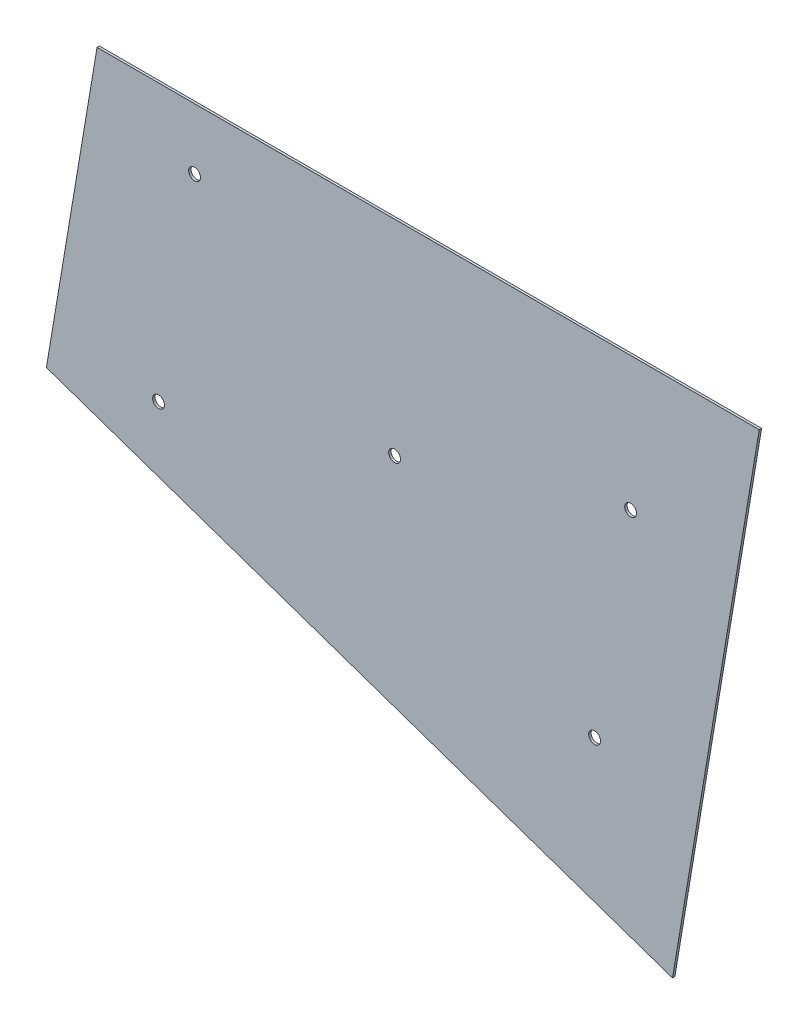
from build123d import *

# Parameters (mm, degrees)
EXTRUDE_1_DEPTH     = 2
SKETCH_2_R          = 5
CUT_EXTRUDE_1_DEPTH = 10


with BuildPart() as part:
    # 草图1 → 凸台-拉伸1 (new body)
    with BuildSketch(Plane.XY):
        Polygon((270.4264573, -50.479352133), (-291.276967283, -50.479352133), (-334.231201576, -307.163734724), (196.869820345, -490.036482017), align=None)
    extrude(amount=EXTRUDE_1_DEPTH)

    # 草图2 → 切除-拉伸1 (cut)
    with BuildSketch(Plane.XY.offset(2)):
        with Locations((-208.545453815, -102.175560394)):
            Circle(SKETCH_2_R)
        with Locations((-239.079260899, -284.638396678)):
            Circle(SKETCH_2_R)
        with Locations((-38.883807069, -224.353404635)):
            Circle(SKETCH_2_R)
        with Locations((130.777839678, -346.531248876)):
            Circle(SKETCH_2_R)
        with Locations((161.311646762, -164.068412591)):
            Circle(SKETCH_2_R)
    extrude(amount=-CUT_EXTRUDE_1_DEPTH, mode=Mode.SUBTRACT)


solid = part.part
